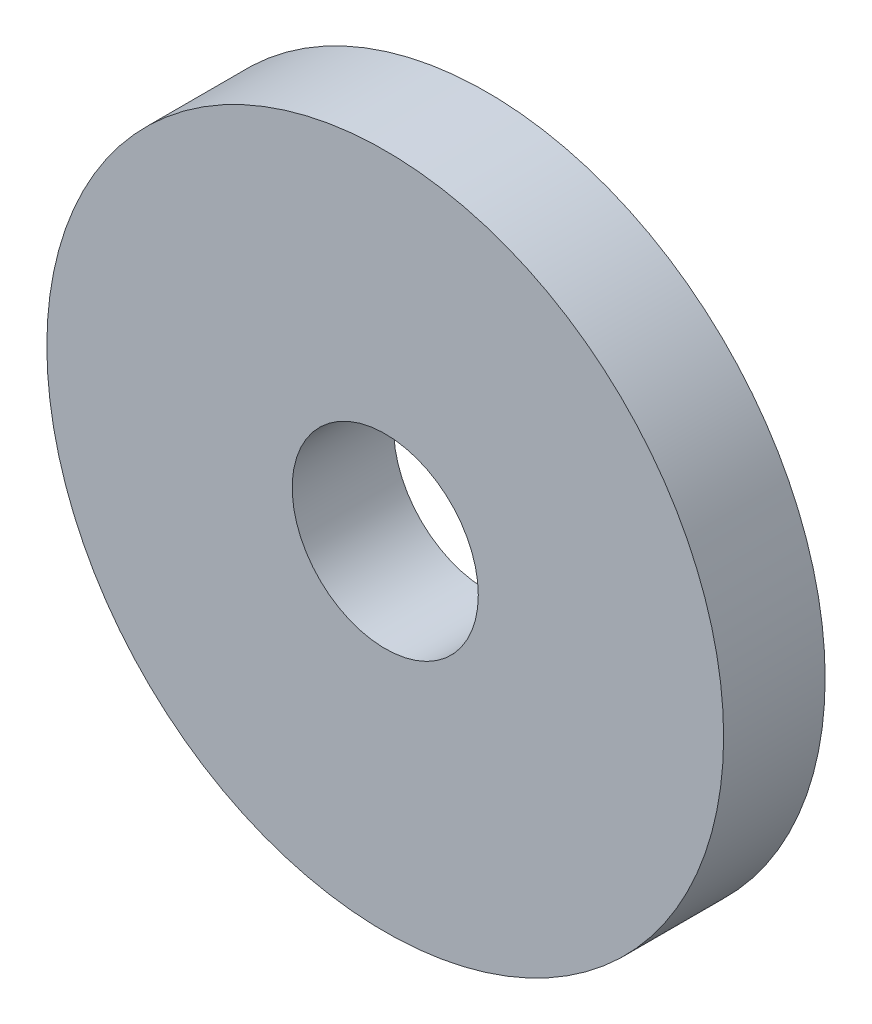
from build123d import *

# Parameters (mm, degrees)
SKETCH1_R           = 40
SKETCH1_R_2         = 11
BOSS_EXTRUDE1_DEPTH = 12


with BuildPart() as part:
    # Sketch1 → Boss-Extrude1 (new body)
    with BuildSketch(Plane.XY):
        Circle(SKETCH1_R)
        Circle(SKETCH1_R_2, mode=Mode.SUBTRACT)
    extrude(amount=BOSS_EXTRUDE1_DEPTH)


solid = part.part
